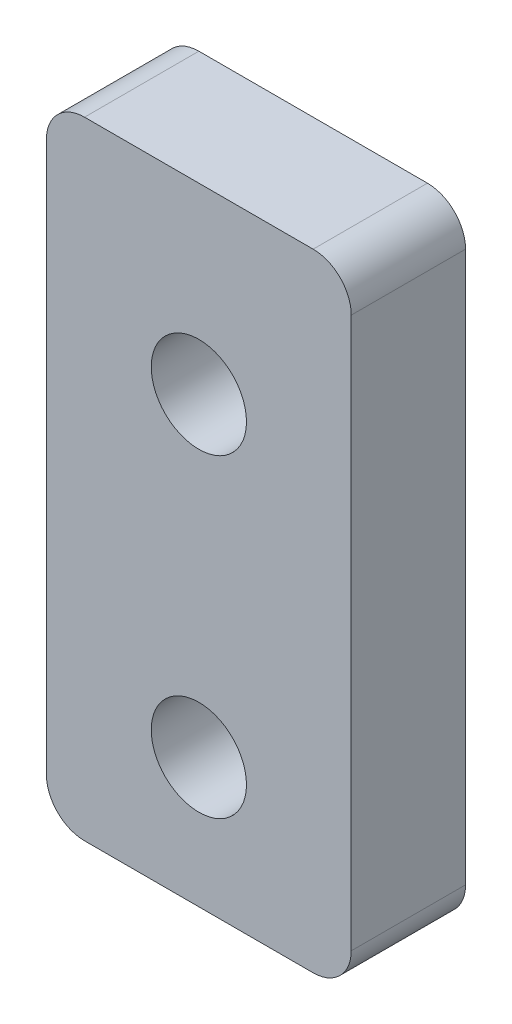
SolidWorks part; units mm, degrees
material "6063-O"
ref_plane "前视基准面" through (0, 0, 0) normal (0, 0, 1) x (1, 0, 0)
ref_plane "上视基准面" through (0, 0, 0) normal (0, 1, 0) x (1, 0, 0)
ref_plane "右视基准面" through (0, 0, 0) normal (1, 0, 0) x (0, 0, -1)
other "Configuration Table"
sketch "草图1" plane through (0, 0, 0) normal (0, 0, 1) x (1, 0, 0)
  line L1 (-4, 13.05) -> (4, 13.05)
  line L2 (-4, 13.05) -> (-4, -3.4)
  line L3 (-4, -3.4) -> (4, -3.4)
  line L4 (4, 13.05) -> (4, -3.4)
  line L5 (-4, 13.05) -> (4, -3.4) construction
  line L6 (-4, -3.4) -> (4, 13.05) construction
  circle A0 centre (0, 0) radius 1.25
  circle A1 centre (0, 8.25) radius 1.25
  point P5 (0, 0)
  point P6 (0, 4.825)
  dimension "D1" = 2.5
  dimension "D2" = 8.25
  dimension "D3" = 3.4
  dimension "D4" = 4.8
  dimension "D5" = 4
extrude "凸台-拉伸1" add sketch "草图1" along normal blind 3
fillet "圆角1" radius 1 4 edges at (-4, -3.4, 1.5) (-4, 13.05, 1.5) (4, 13.05, 1.5) (4, -3.4, 1.5)
